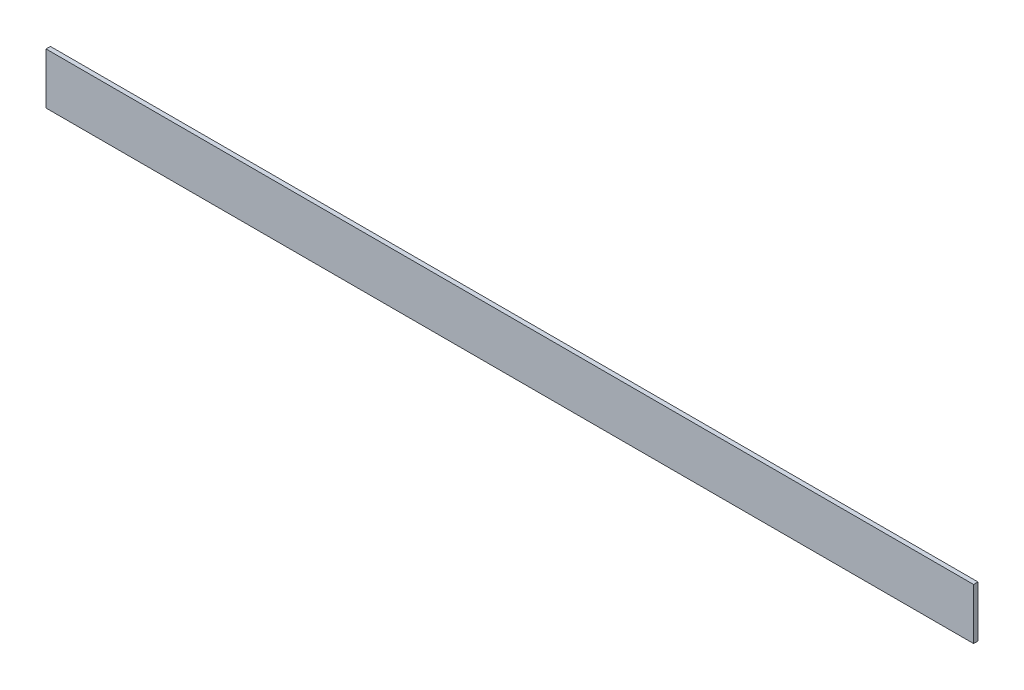
from build123d import *

# Parameters (mm, degrees)
SKETCH_1_W      = 634
SKETCH_1_H      = 35
EXTRUDE_1_DEPTH = 3


with BuildPart() as part:
    # 草图1 → 凸台-拉伸1 (new body)
    with BuildSketch(Plane.XY):
        Rectangle(SKETCH_1_W, SKETCH_1_H)
    extrude(amount=EXTRUDE_1_DEPTH)


solid = part.part
